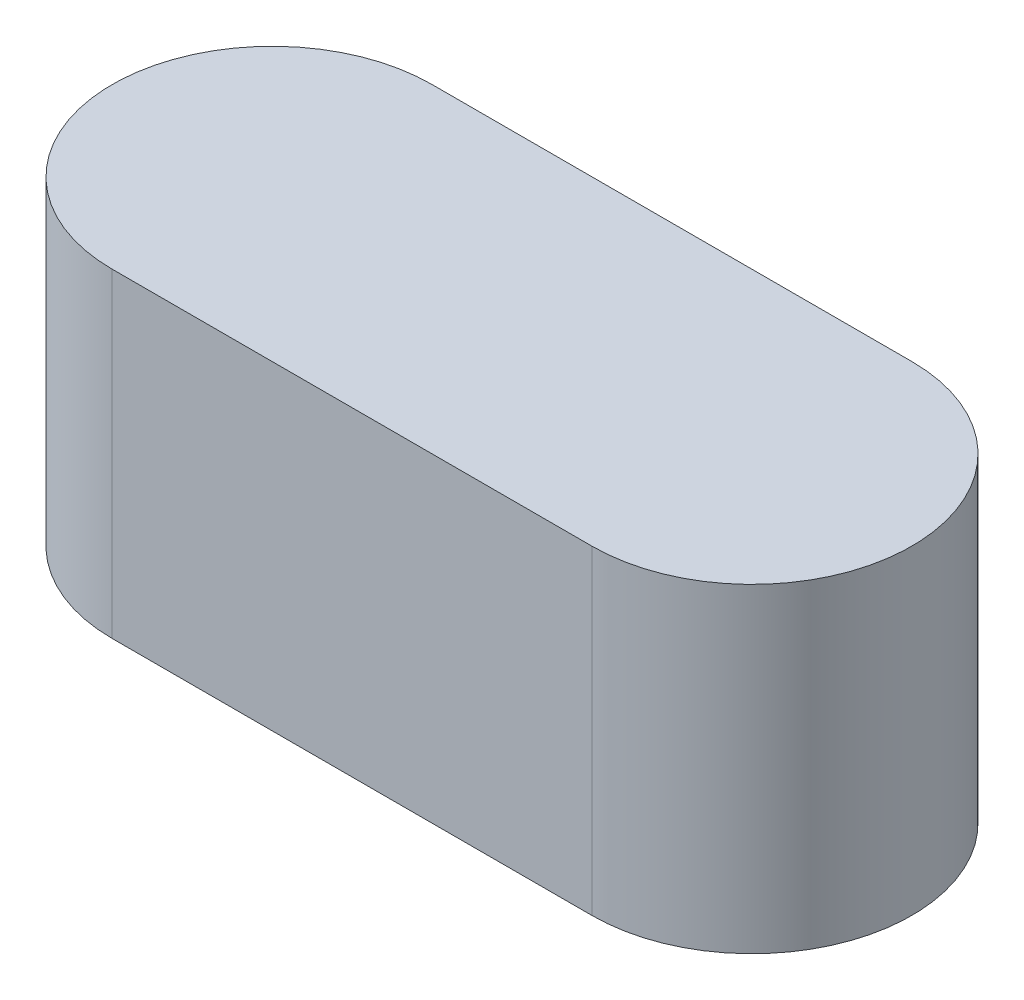
from build123d import *

# Parameters (mm, degrees)
BOSS_EXTRUDE1_DEPTH = 100


with BuildPart() as part:
    # Sketch1 → Boss-Extrude1 (new body)
    with BuildSketch(Plane(origin=(0, 0, 0), x_dir=(1, 0, 0), z_dir=(0, 1, 0))):
        with BuildLine():
            Line((-75, 50), (75, 50))
            ThreePointArc((75, 50), (125, 0), (75, -50))
            Line((75, -50), (-75, -50))
            ThreePointArc((-75, -50), (-125, 0), (-75, 50))
        make_face()
    extrude(amount=BOSS_EXTRUDE1_DEPTH)


solid = part.part
